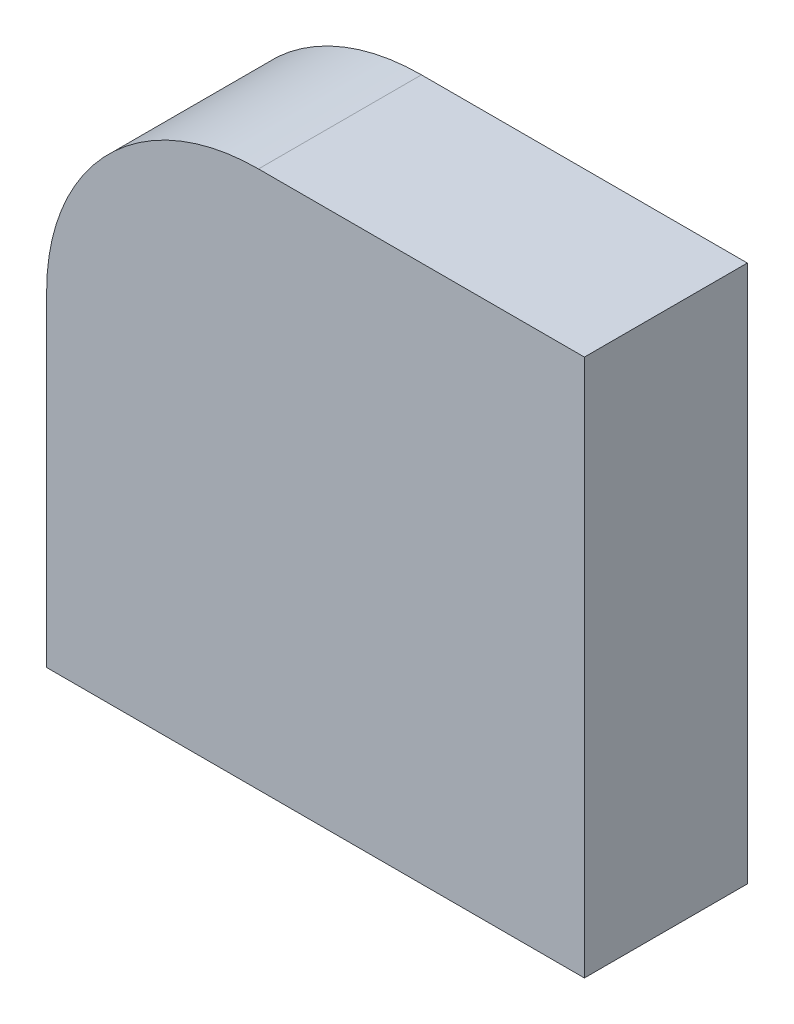
SolidWorks part; units mm, degrees
material "Q235A"
ref_plane "Front Plane" through (0, 0, 0) normal (0, 0, 1) x (1, 0, 0)
ref_plane "Top Plane" through (0, 0, 0) normal (0, 1, 0) x (1, 0, 0)
ref_plane "Right Plane" through (0, 0, 0) normal (1, 0, 0) x (0, 0, -1)
sketch "Sketch1" plane through (0, 0, 0) normal (0, 0, 1) x (1, 0, 0)
  line L0 (0, 0) -> (0, 40)
  line L1 (0, 40) -> (40, 40)
  line L2 (40, 40) -> (40, 0)
  line L5 (40, 0) -> (0, 0)
  dimension "D1" = 40
  dimension "D2" = 40
extrude "Boss-Extrude1" add sketch "Sketch1" along normal blind 10
fillet "Fillet1" radius 20 1 edges at (0, 40, 5)
sketch "Sketch2" plane through (0, 0, 0) normal (0, 0, -1) x (-1, 0, 0)
  line L0 (-40, 40) -> (-20, 40) construction
  line L1 (0, 20) -> (0, 0) construction
  line L2 (-40, 40) -> (-20, 40)
  line L3 (0, 20) -> (0, 0)
  line L4 (-40, 33) -> (-20, 33)
  line L5 (-7, 20) -> (-7, 0)
  line L6 (-40, 33) -> (-40, 40)
  line L7 (-7, 0) -> (0, 0)
  arc A0 (0, 20) -> (-20, 40) centre (-20, 20) ccw construction
  arc A1 (0, 20) -> (-20, 40) centre (-20, 20) ccw
  arc A2 (-7, 20) -> (-20, 33) centre (-20, 20) ccw
  dimension "D1" = 7
extrude "Cut-Extrude1" cut sketch "Sketch2" against normal through all
